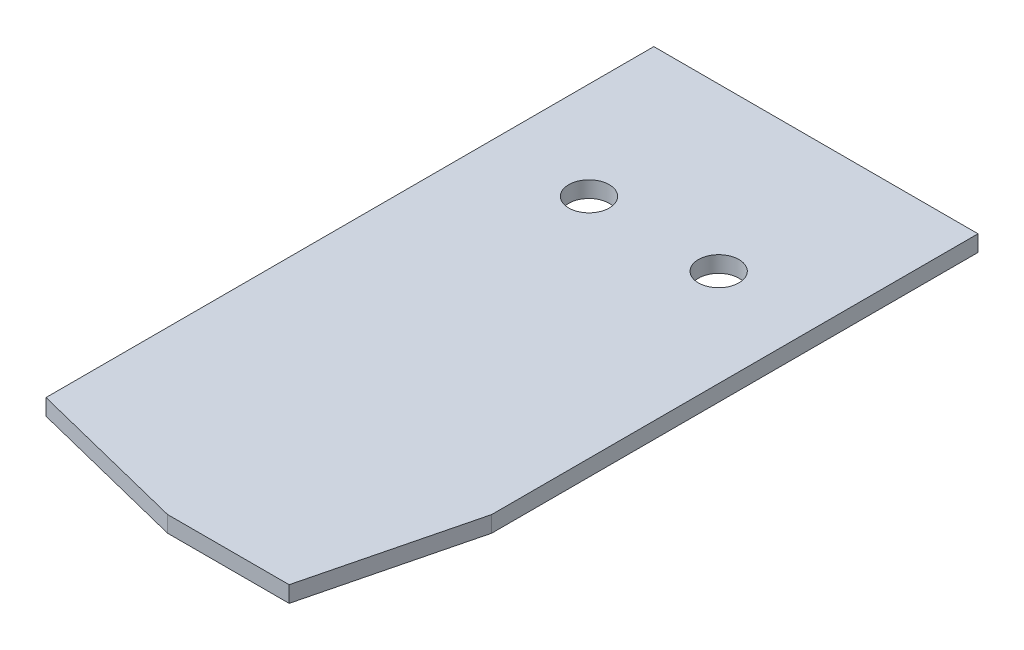
SolidWorks part; units mm, degrees
ref_plane "Front Plane" through (0, 0, 0) normal (0, 0, 1) x (1, 0, 0)
ref_plane "Top Plane" through (0, 0, 0) normal (0, 1, 0) x (1, 0, 0)
ref_plane "Right Plane" through (0, 0, 0) normal (1, 0, 0) x (0, 0, -1)
sketch "Sketch1" plane through (0, 0, 0) normal (0, 1, 0) x (1, 0, 0)
  line L1 (-20, 40) -> (20, 40)
  line L2 (-20, 40) -> (-20, -40)
  line L3 (-20, -40) -> (20, -40)
  line L4 (20, 40) -> (20, -40)
  line L5 (-20, 40) -> (20, -40) construction
  line L6 (-20, -40) -> (20, 40) construction
  point P0 (0, 0)
  dimension "D1" = 40
  dimension "D2" = 80
extrude "Boss-Extrude1" add sketch "Sketch1" along normal blind 2
sketch "Sketch2" plane through (0, 0, 0) normal (0, -1, 0) x (1, 0, 0)
  circle A0 centre (8, -20) radius 2.5
  circle A1 centre (-8, -20) radius 2.5
  dimension "D1" = 5
extrude "Cut-Extrude1" cut sketch "Sketch2" against normal blind 10
chamfer "Chamfer1" distance 5 distance2 20 2 edges at (20, 1, 40) (-20, 1, 40)
